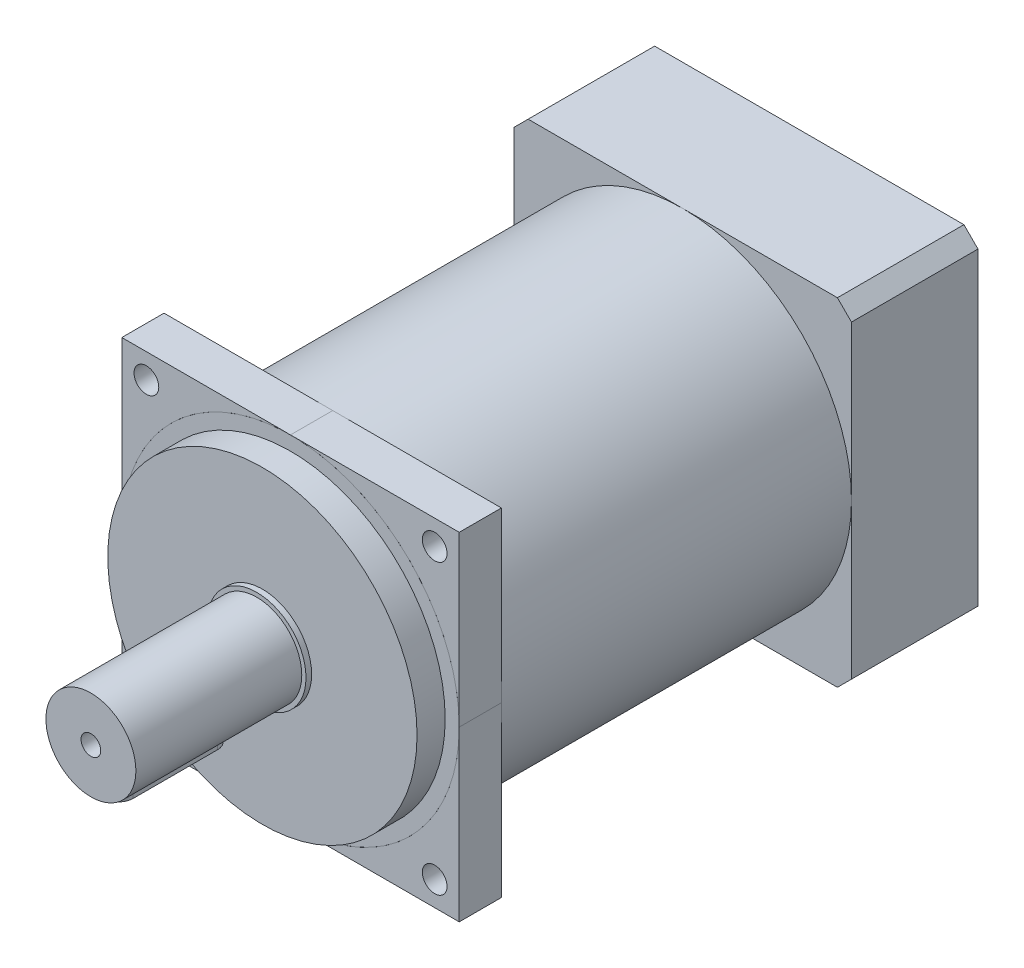
SolidWorks part; units mm, degrees
ref_plane "Front Plane" through (0, 0, 0) normal (0, 0, 1) x (1, 0, 0)
ref_plane "Top Plane" through (0, 0, 0) normal (0, 1, 0) x (1, 0, 0)
ref_plane "Right Plane" through (0, 0, 0) normal (1, 0, 0) x (0, 0, -1)
sketch "Sketch1" plane through (0, 0, 0) normal (0, 0, 1) x (1, 0, 0)
  line L1 (0, 0) -> (120, 0)
  line L2 (0, 0) -> (0, -120)
  line L3 (0, -120) -> (120, -120)
  line L4 (120, 0) -> (120, -120)
  dimension "D1" = 120
  dimension "D2" = 120
extrude "Extrude1" add sketch "Sketch1" along normal blind 45
sketch "Sketch2" plane through (0, 0, 45) normal (0, 0, 1) x (1, 0, 0)
  line L0 (0, 0) -> (0, -120) construction
  line L1 (0, -120) -> (120, -120) construction
  circle A0 centre (60, -60) radius 60
  dimension "D1" = 120
  dimension "D2" = 60
  dimension "D3" = 60
extrude "Extrude2" add sketch "Sketch2" along normal blind 139.5
sketch "Sketch3" plane through (0, 0, 184.5) normal (0, 0, 1) x (1, 0, 0)
  circle A0 centre (60, -60) radius 55
  dimension "D1" = 110
extrude "Extrude3" add sketch "Sketch3" along normal blind 10
sketch "Sketch4" plane through (0, 0, 194.5) normal (0, 0, 1) x (1, 0, 0)
  circle A0 centre (60, -60) radius 17.5
  dimension "D1" = 35
extrude "Extrude4" add sketch "Sketch4" along normal blind 2
sketch "Sketch5" plane through (0, 0, 196.5) normal (0, 0, 1) x (1, 0, 0)
  circle A0 centre (60, -60) radius 16
  dimension "D1" = 32
extrude "Extrude5" add sketch "Sketch5" along normal blind 59
sketch "Sketch6" plane through (0, 0, 184.5) normal (0, 0, 1) x (1, 0, 0)
  circle A0 centre (60, -60) radius 50 construction
  dimension "D1" = 100
chamfer "Chamfer1" distance 5 angle 45 4 edges at (120, -120, 22.5) (120, 0, 22.5) (0, 0, 22.5) (0, -120, 22.5)
hole_wizard "M8x1.0 Tapped Hole1" positions "Sketch17" profile "Sketch16" tap size "M8x1.0" standard "ISO"
sketch "Sketch17" plane through (0, 0, 255.5) normal (0, 0, 1) x (1, 0, 0)
  point P1 (60, -60)
sketch "Sketch16" plane through (60, -60, 255.5) normal (1, 0, 0) x (0, -1, 0)
  line L0 (0, 0) -> (0, 21.103)
  line L1 (0, 21.103) -> (3.5, 19)
  line L2 (3.5, 19) -> (3.5, 0)
  line L5 (3.5, 0) -> (0, 0)
  line L10 (0, 21.103) -> (-3.5, 19) construction
  line L11 (0, -6.35) -> (0, 107.95) construction
  dimension "蹟恇謂郰芛眻噤" = 7
  dimension "蹟恇謂郰芛旮僅" = 19
  dimension "絳芛褒僅" = 118
cosmetic thread "Cosmetic Thread10" parameters "D1"=16, "D2"=8
ref_plane "Plane1" through (0, -76, 0) normal (0, -1, 0) x (1, 0, 0)
sketch "Sketch18" plane through (0, -76, 0) normal (0, -1, 0) x (1, 0, 0)
  line L0 (55, 245.5) -> (55, 215.5)
  line L1 (65, 245.5) -> (65, 215.5)
  line L5 (76, 255.5) -> (44, 255.5) construction
  line L8 (60, 255.5) -> (60, 196.5) construction
  arc A0 (55, 245.5) -> (65, 245.5) centre (60, 245.5) cw
  arc A1 (55, 215.5) -> (65, 215.5) centre (60, 215.5) ccw
  dimension "D7" = 5
  dimension "D8" = 5
  dimension "D1" = 30
  dimension "D2" = 30
  dimension "D3" = 10
  dimension "D4" = 10
  dimension "D5" = 10
  dimension "D6" = 5
extrude "Extrude6" add sketch "Sketch18" along normal blind 3
sketch "Sketch19" plane through (0, 0, 0) normal (-1, 0, 0) x (0, 0, 1)
  line L0 (184.5, 0) -> (45, 0) construction
  line L1 (0, -5) -> (0, -115) construction
  circle A0 centre (10, -20) radius 5
  dimension "D1" = 10
  dimension "D2" = 20
  dimension "D3" = 10
extrude "Cut-Extrude1" cut sketch "Sketch19" against normal blind 10
sketch "Sketch20" plane through (0, 0, 0) normal (0, 0, -1) x (-1, 0, 0)
  line L0 (-60, 0) -> (-60, -120) construction
  line L1 (-115, 0) -> (-5, 0) construction
  line L2 (-5, -120) -> (-115, -120) construction
  line L3 (-120, -60) -> (0, -60) construction
  line L4 (-120, -115) -> (-120, -5) construction
  circle A0 centre (-60, -60) radius 55
  dimension "D1" = 110
extrude "Cut-Extrude2" cut sketch "Sketch20" against normal blind 7
hole_wizard "M8 Tapped Hole1" positions "Sketch22" profile "Sketch21" tap size "M8" standard "GB"
sketch "Sketch22" plane through (0, 0, 0) normal (0, 0, -1) x (-1, 0, 0)
  line L0 (-60, -5) -> (-60, -115) construction
  line L2 (-111.2652, -8.7348) -> (-60, -60) construction
  circle A0 centre (-60, -60) radius 55 construction
  point P0 (-111.2652, -8.7348)
  dimension "D1" = 72.5
  dimension "D2" = 45
sketch "Sketch21" plane through (111.2652, -8.7348, 0) normal (1, 0, 0) x (0, 1, 0)
  line L0 (0, 0) -> (0, 21.7929)
  line L1 (0, 21.7929) -> (3.4, 19.75)
  line L2 (3.4, 19.75) -> (3.4, 0)
  line L5 (3.4, 0) -> (0, 0)
  line L10 (0, 21.7929) -> (-3.4, 19.75) construction
  line L11 (0, -6.35) -> (0, 107.95) construction
  dimension "螺纹孔钻头直径" = 6.8
  dimension "螺纹孔钻头深度" = 19.75
  dimension "导头角度" = 118
cosmetic thread "Cosmetic Thread11" parameters "D1"=16, "D2"=8
pattern_circular "CirPattern1" count 4 over 360 about axis through (60, -60, 0) along (0, 0, 1) of "M8 Tapped Hole1"
sketch "Sketch23" plane through (0, 0, 184.5) normal (0, 0, 1) x (1, 0, 0)
  line L1 (0, 0) -> (120, 0)
  line L2 (0, 0) -> (0, -120)
  line L3 (0, -120) -> (120, -120)
  line L4 (120, 0) -> (120, -120)
  line L5 (0, 0) -> (120, -120) construction
  line L6 (0, -120) -> (120, 0) construction
  circle A0 centre (60, -60) radius 60
  circle M1 centre (60, -60) radius 60
  dimension "D3" = 120
  dimension "D1" = 120
  dimension "D2" = 120
extrude "Boss-Extrude1" add sketch "Sketch23" against normal blind 15 separate body contours L4 L1 M1 | L1 L2 M1 | L2 L3 M1 | L4 L3 M1
sketch "Sketch24" plane through (0, 0, 184.5) normal (0, 0, 1) x (1, 0, 0)
  line L0 (60, -5) -> (60, -115) construction
  line L1 (8.7348, -8.7348) -> (60, -60) construction
  circle A0 centre (8.7348, -8.7348) radius 4.4
  circle A1 centre (60, -60) radius 55 construction
  circle A2 centre (60, -60) radius 55 construction
  dimension "D2" = 8.8
  dimension "D1" = 72.5
  dimension "D3" = 45
extrude "Cut-Extrude3" cut sketch "Sketch24" against normal blind 15
pattern_circular "CirPattern2" count 4 over 360 about axis through (60, -60, 0) along (0, 0, 1) of "Cut-Extrude3"
